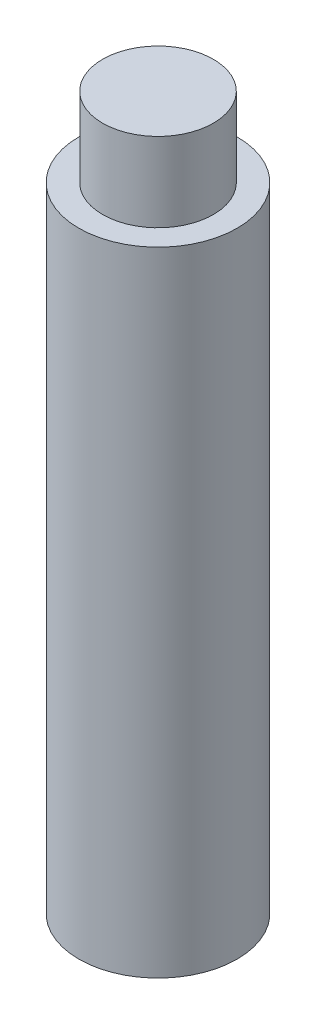
from build123d import *

# Parameters (mm, degrees)
SKETCH1_R           = 10
BOSS_EXTRUDE1_DEPTH = 5
SKETCH2_R           = 10
BOSS_EXTRUDE2_DEPTH = 75
SKETCH3_R           = 7
BOSS_EXTRUDE3_DEPTH = 10


with BuildPart() as part:
    # Sketch1 → Boss-Extrude1 (new body)
    with BuildSketch(Plane(origin=(0, 0, 0), x_dir=(1, 0, 0), z_dir=(0, 1, 0))):
        with Locations(Location((0, 0, 0), (0, 0, 270))):
            Circle(SKETCH1_R)
    extrude(amount=BOSS_EXTRUDE1_DEPTH)

    # Sketch2 → Boss-Extrude2 (add)
    with BuildSketch(Plane(origin=(0, 5, 0), x_dir=(1, 0, 0), z_dir=(0, 1, 0))):
        with Locations(Location((0, 0, 0), (0, 0, 270))):
            Circle(SKETCH2_R)
    extrude(amount=BOSS_EXTRUDE2_DEPTH)

    # Sketch3 → Boss-Extrude3 (add)
    with BuildSketch(Plane(origin=(0, 80, 0), x_dir=(1, 0, 0), z_dir=(0, 1, 0))):
        with Locations(Location((0, 0, 0), (0, 0, 270))):
            Circle(SKETCH3_R)
    extrude(amount=BOSS_EXTRUDE3_DEPTH)


solid = part.part
